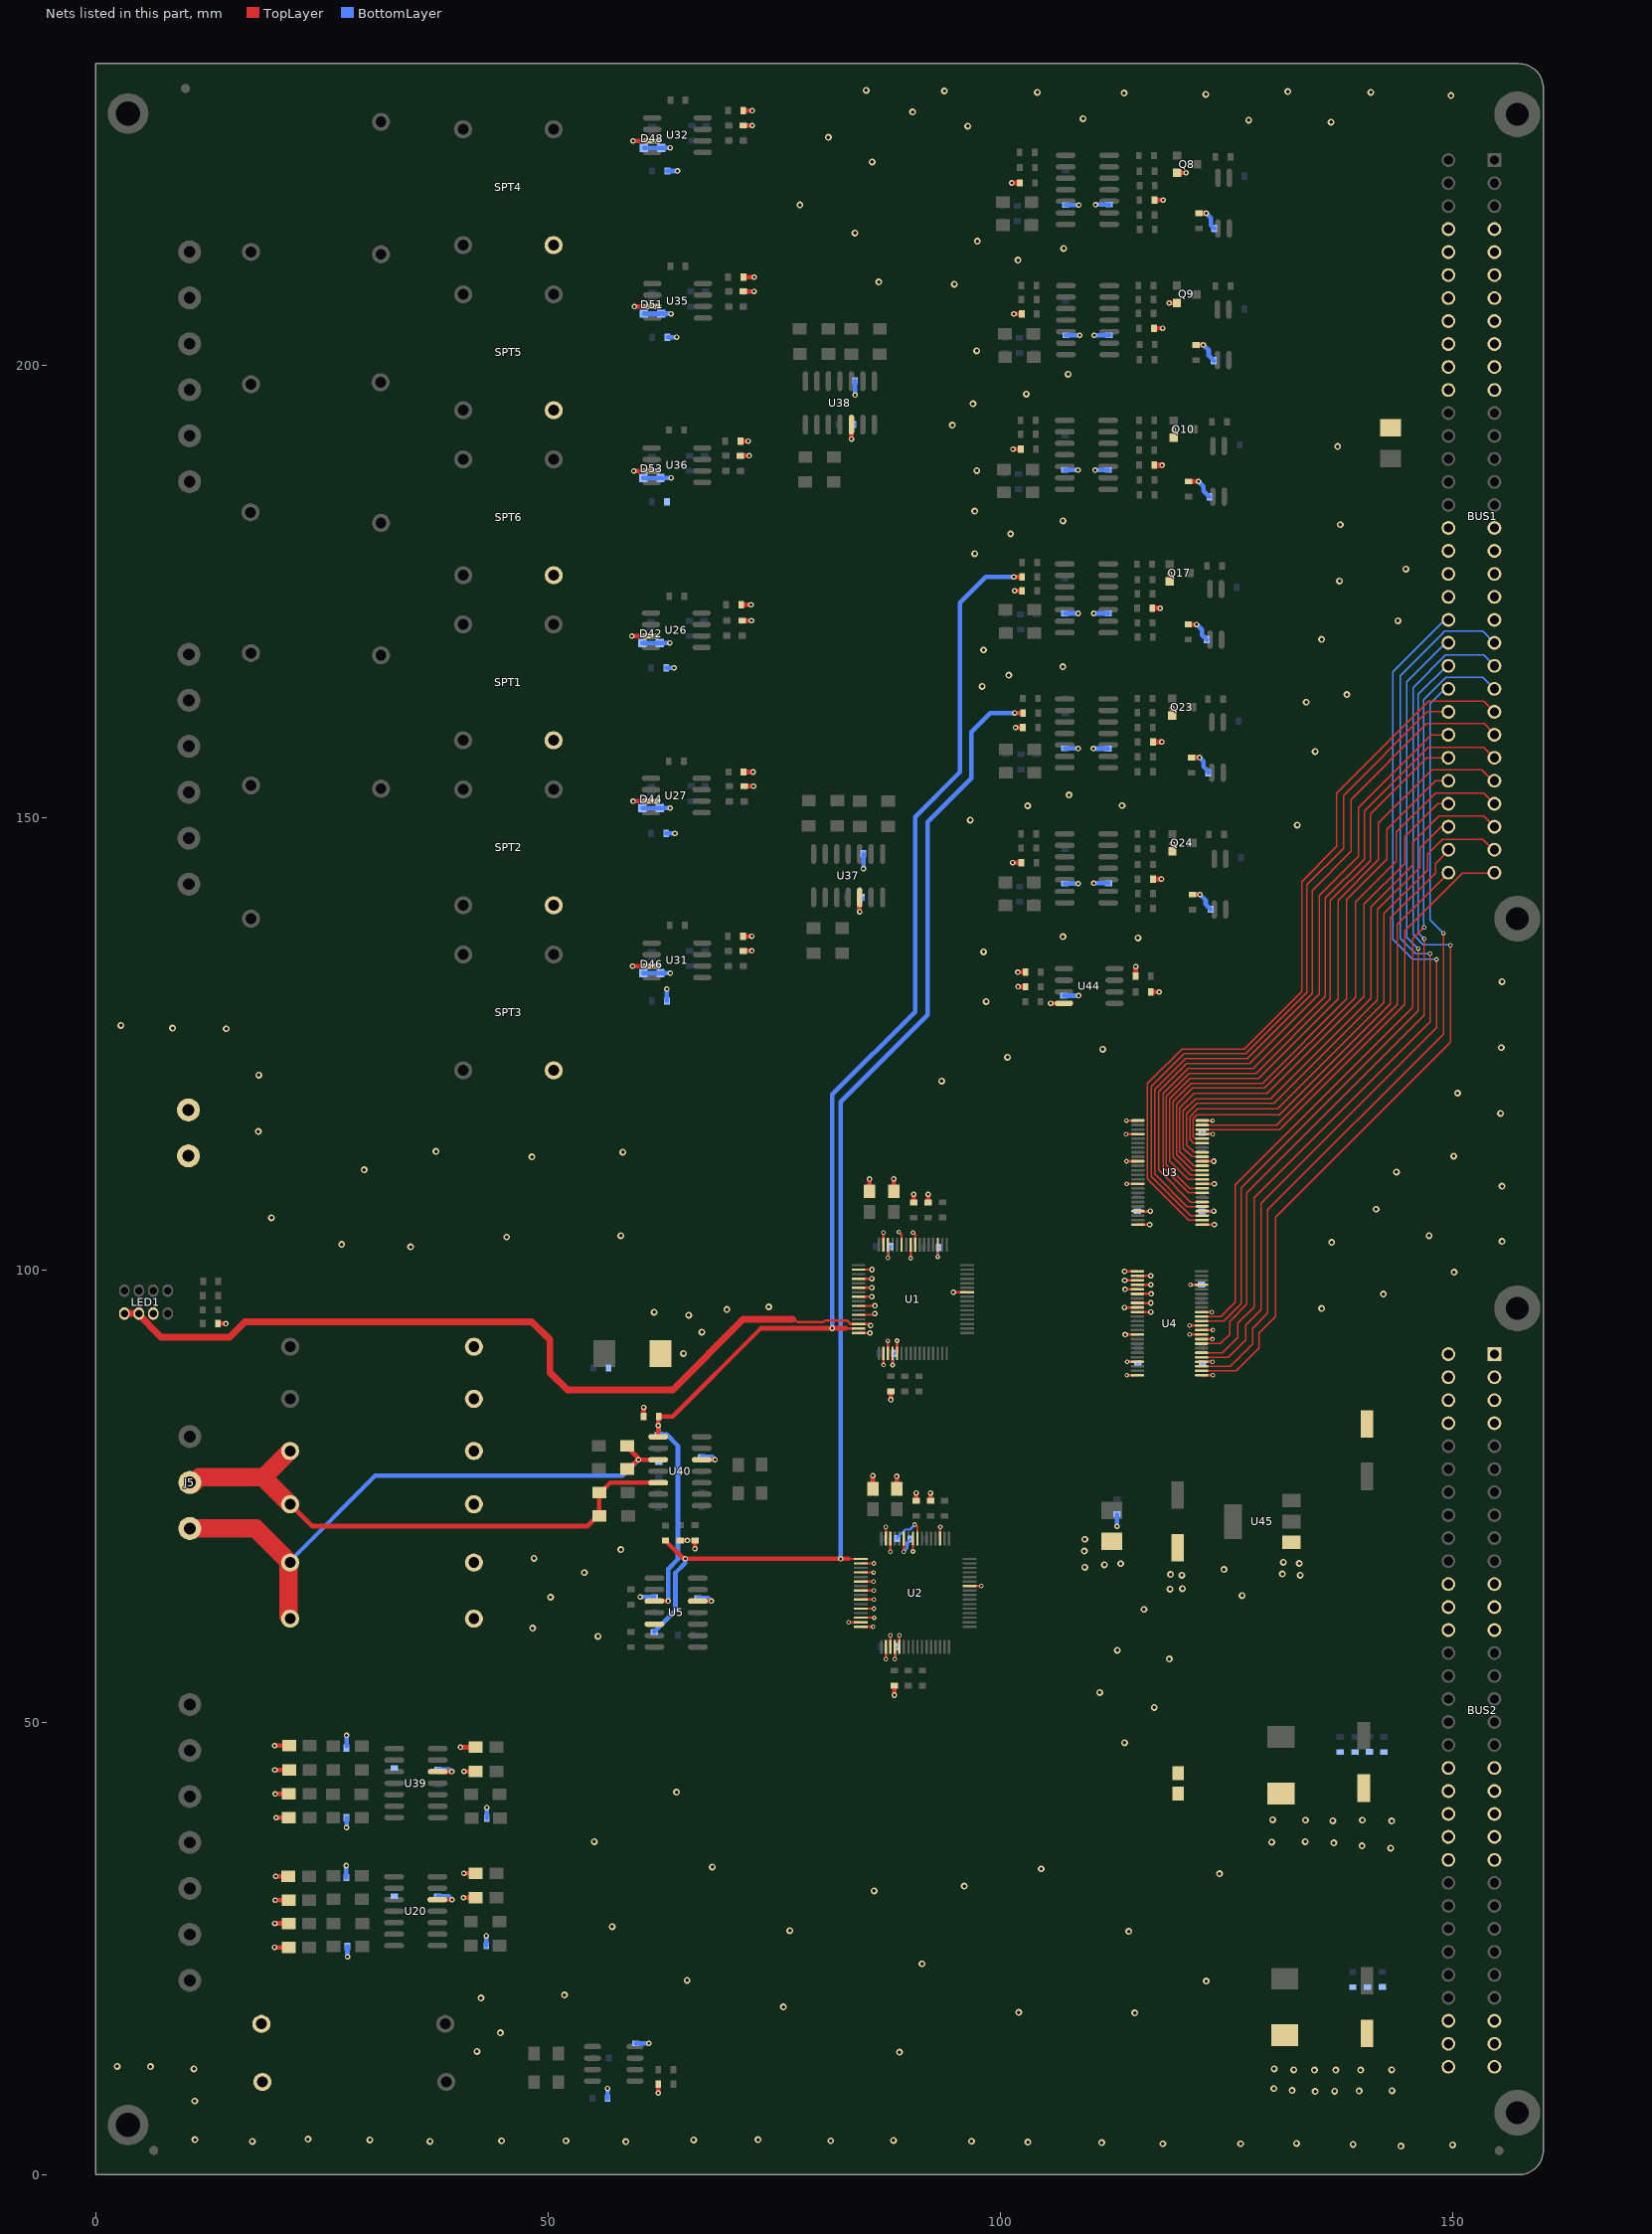
[diagram p0: the nets of this part, all layers, seen from the top]
# Altium PCB MISC80584.PCBDoc (part 4 of 7)
Units mm, origin at the board's own origin, x right, y up, seen from the top; angles counter-clockwise.
Board outline 160.02 x 233.3 mm, 4 copper layers (TopLayer, GND, POWER, BottomLayer); 386 components, 266 nets, 1374 pads, 640 vias.

## Via types
v1: diameter 0.61, hole 0.305, TopLayer to BottomLayer, 342 vias
v2: diameter 0.762, hole 0.381, TopLayer to BottomLayer, 197 vias
v3: diameter 0.508, hole 0.254, TopLayer to BottomLayer, 101 vias

## Nets (pads, with @x,y where several pads share a name; then routed paths per layer and width w, separated by ;. In a path a pad name is that pad's centre, name@x,y a point inside that pad or via, vN(x,y) a via of type N, cw(c..) or ccw(c..) an arc to the next point about the centre after c; other vN are vias at no path point) (continued)
AGND: BUS2.A11 BUS2.A12 BUS2.A13 BUS2.A19 BUS2.A20 BUS2.A21 BUS2.A22 BUS2.A23 BUS2.A30 BUS2.A31 BUS2.A32 BUS2.C11 BUS2.C12 BUS2.C13 BUS2.C19 BUS2.C20 BUS2.C21 BUS2.C22 BUS2.C23 BUS2.C30 BUS2.C31 BUS2.C32 C9.1 C10.1 C11.1 C12.1 C13.1 C14.1 C20.1 C21.1 C23.1 C27.1 C85.1 C93.1 C101.1 C119.2 C120.2 C121.1 C122.1 C123.1 C124.1 C126.1 C136.1 C139.1 C146.2 C147.2 C148.2 C149.1 C173.1 C174.2 C175.2 C176.1 C177.2 C178.1 C179.1 C180.2 C181.2 C182.1 C183.1 C184.2 C192.1 C193.2 C194.1 C195.2 C196.2 C197.1 C204.1 C205.1 C206.2 C215.2 C216.1 C217.1 C218.2 C219.1 C220.1 C224.2 C230.1 C231.2 C232.2 C233.1 C234.2 C235.1 C238.1 C239.2 C240.2 C249.2 C251.1 C252.2 C253.1 C254.2 C255.2 C256.1 C257.1 C261.1 C262.2 CT2.2 CT3.1 CT4.2 CT7.2 CT13.1 D42.1 D42.2 D44.1 D44.2 D46.1 D46.2 D48.1 D48.2 D51.1 D51.2 D53.1 D53.2 J4.1 J4.2 L1.2 LED1.6 Q8.E Q9.E Q10.E Q17.E Q23.E Q24.E R1.1 R2.1 R3.1 R4.1 R6.1 R7.1 R8.1 R9.1 R23.2 R24.2 R25.2 R26.2 R27.2 R29.2 R30.2 R31.2 R32.2 R35.2 R36.2 R38.2 R341.2 R399.2 R400.2 R401.2 R423.2 R430.2 R431.2 R435.2 R437.2 R438.2 R444.2 R445.2 R446.2 SPT1.2 SPT2.2 SPT3.2 SPT4.2 SPT5.2 SPT6.2 U1.43 U1.46 U1.47 U2.43 U2.46 U2.47 U5.5 U5.12 U20.12 U26.3 U27.3 U31.3 U32.3 U35.3 U36.3 U37.12 U38.12 U39.12 U40.12 U44.4 | length 161.6
  TopLayer w0.254: U1.47@87.089,102.805 v3(87.089,104.157) ; U2.47@87.343,70.344 v3(87.343,71.636) ; v3(87.589,101.355) U1.46@87.589,102.805 ; v3(87.843,68.894) U2.46@87.843,70.344 ; v3(88.798,104.191) 89.089,103.901 U1.43@89.089,102.805 ; v3(89.343,68.896) U2.43@89.343,70.344
  TopLayer w0.508: R341.2@13.513,94.082 v1(14.402,94.082) ; v1(19.787,25.171) R30.2@21.336,25.171 ; v1(19.787,47.447) R24.2@21.387,47.447 ; v1(19.812,27.813) R31.2@21.336,27.813 ; v1(19.812,44.755) R23.2@21.387,44.755 ; v1(19.863,30.378) R25.2@21.336,30.378 ; v1(19.863,42.113) R27.2@21.361,42.113 ; v1(19.914,33.02) R26.2@21.311,33.02 ; v1(19.939,39.497) R29.2@21.361,39.497 ; U20.12@37.782,30.429 v1(39.395,30.429) ; U39.12@37.808,44.577 v1(39.37,44.577) ; v1(40.335,47.269) R32.2@42.012,47.269 ; v1(40.665,30.658) R36.2@42.012,30.658 ; v1(40.691,33.35) R38.2@42.012,33.35 ; v1(40.716,44.602) R35.2@42.012,44.602 ; v1(59.258,170.078) U26.3@61.392,170.078 ; v1(59.36,133.604) U31.3@61.468,133.604 ; v1(59.411,151.816) U27.3@61.392,151.816 ; v1(59.411,224.79) U32.3@61.519,224.79 ; v1(59.487,188.316) U36.3@61.468,188.316 ; v1(59.563,206.477) U35.3@61.544,206.477 ; C10.1@60.579,83.82 v1(60.579,84.836) ; v1(62.205,9.068) C9.1@62.205,10.058 ; C11.1@64.618,70.129 v1(65.405,70.129) ; v1(66.243,69.215) C14.1@66.243,70.129 ; U5.12@66.56,63.424 v1(68.047,63.424) ; U40.12@66.992,79.045 v1(68.478,79.045) ; C136.1@71.272,189.992 v1(72.238,189.992) ; C181.2@71.272,191.618 v1(72.136,191.618) ; C180.2@71.374,173.533 v1(72.441,173.533) ; C85.1@71.476,171.78 v1(72.492,171.78) ; C178.1@71.552,136.906 v1(72.542,136.906) ; C101.1@71.577,135.28 v1(72.542,135.28) ; C139.1@71.577,226.492 v1(72.568,226.492) ; C183.1@71.577,228.117 v1(72.568,228.117) ; C126.1@71.603,208.153 v1(72.771,208.153) ; C184.2@71.603,209.728 v1(72.796,209.728) ; C179.1@71.628,155.042 v1(72.669,155.042) ; C93.1@71.679,153.467 v1(72.72,153.467) ; v1(83.541,191.846) U38.12@83.541,193.434 ; v1(84.455,139.598) U37.12@84.455,141.186 ; C121.1@85.547,108.712 v1(85.547,110.058) ; C123.1@85.903,75.844 v1(85.903,77.292) ; C122.1@88.214,108.712 v1(88.214,110.084) ; C124.1@88.544,75.844 v1(88.544,77.216) ; v1(101.27,220.142) R399.2@102.159,220.142 ; v1(101.371,145.034) R431.2@102.311,145.034 ; v1(101.397,190.729) R401.2@102.26,190.729 ; v1(101.498,205.664) R400.2@102.362,205.664 ; v1(101.575,175.057) R423.2@102.413,175.057 ; v1(101.676,159.969) R430.2@102.489,159.969 ; v1(101.93,132.918) C146.2@102.794,132.918 ; v1(101.956,131.318) C147.2@102.794,131.318 ; v1(105.562,129.489) U44.4@107.036,129.489 ; C149.1@114.96,132.486 v1(114.96,133.528) ; C148.2@116.637,130.734 v1(117.577,130.734) ; R438.2@116.992,204.089 v1(117.958,204.089) ; R437.2@117.043,218.237 v1(118.008,218.237) ; v1(118.669,206.883) Q9.E@119.507,206.883 ; Q17.E@118.72,176.098 v1(118.72,176.962) ; Q23.E@118.999,161.265 v1(118.999,162.077) ; Q24.E@119.024,146.279 v1(119.024,147.117) ; Q10.E@119.151,191.973 v1(119.151,192.837) ; Q8.E@119.558,221.259 v1(120.523,221.259)
  TopLayer w0.635: R444.2@116.789,173.152 v1(117.678,173.152) ; R446.2@116.865,143.205 v1(117.805,143.205) ; R445.2@116.865,158.369 v1(117.856,158.369) ; R435.2@117.018,188.951 v1(117.881,188.951)
  BottomLayer w0.305: v3@87.579,101.448 87.579,102.286 C119.2@87.884,102.591 ; v3@89.332,68.91 89.687,69.266 89.687,69.901 C120.2@90.068,70.282
  BottomLayer w0.508: C13.1@27.711,32.868 v1(27.711,34.188) ; v1(27.737,38.405) C20.1@27.737,39.497 ; C12.1@27.737,47.396 v1(27.737,48.59) ; v1(27.838,24.105) C21.1@27.838,25.273 ; C192.1@37.821,30.785 39.04,30.785 v1@39.345,30.48 ; C194.1@37.846,44.806 39.141,44.806 v1@39.319,44.628 ; C27.1@43.18,25.349 v1(43.18,26.441) ; C23.1@43.231,39.446 v1(43.231,40.615) ; C195.2@56.591,8.484 v1(56.591,9.576) ; C220.1@59.741,14.554 v1(61.138,14.554) ; v1(60.198,63.881) C177.2@61.747,63.881 ; D44.2@60.452,151.054 v1(63.5,151.054) ; D42.2@60.452,169.316 v1(63.475,169.316) ; D46.2@60.528,132.817 v1(63.525,132.817) ; D53.2@60.528,187.554 v1(63.627,187.554) ; D51.2@60.604,205.689 D51.1@62.509,205.689 62.662,205.689 v1(63.602,205.689) ; D48.2@60.604,224.028 D48.1@62.509,224.028 62.636,224.028 v1(63.5,224.028) ; C254.2@63.068,148.26 v1(64.033,148.26) ; C252.2@63.068,166.548 v1(63.932,166.548) ; C253.1@63.144,129.743 v1(63.144,131.064) ; C261.1@63.195,221.463 v1(64.313,221.463) ; C251.1@63.221,203.098 v1(64.237,203.098) ; C196.2@66.573,63.754 67.666,63.754 v1@67.97,63.449 ; C197.1@66.98,79.35 68.148,79.35 v1@68.428,79.07 ; v1(83.541,191.846) 83.541,193.116 C240.2@83.845,193.421 ; v1(83.947,196.698) C224.2@83.947,198.272 ; v1(84.455,139.598) 84.455,140.741 C262.2@84.76,141.046 ; v1(84.861,144.348) C233.1@84.861,145.999 ; C216.1@107.036,130.327 v1(108.661,130.327) ; C217.1@107.112,157.658 108.585,157.658 v1(108.61,157.632) ; C232.2@107.112,188.417 v1(108.585,188.417) ; C231.2@107.137,142.723 v1(108.61,142.723) ; C218.2@107.137,172.568 v1(108.61,172.568) ; C215.2@107.213,217.703 v1(108.687,217.703) ; C219.1@107.264,203.302 v1(108.788,203.302) ; v1(110.287,157.632) C238.1@111.912,157.632 ; v1(110.338,142.748) C255.2@111.963,142.748 ; v1(110.338,172.568) C256.1@111.938,172.568 ; v1(110.388,203.302) C193.2@112.039,203.302 ; v1(110.49,188.392) 110.515,188.417 C239.2@111.938,188.417 ; v1(110.515,217.729) 110.541,217.754 C257.1@112.039,217.754
  other v2: 144.272,3.2 149.987,3.327 138.989,3.378 117.958,3.454 126.568,3.454 132.74,3.505 111.201,3.581 103.048,3.632 58.598,3.683 17.323,3.708 36.957,3.708 96.825,3.734 44.882,3.785 51.994,3.785 81.255,3.785 88.189,3.835 30.328,3.886 66.116,3.886 10.973,3.912 73.228,3.912 23.47,3.962 10.947,8.179 134.798,9.246 136.957,9.271 139.675,9.296 143.281,9.322 132.258,9.347 130.251,9.55 134.722,11.608 137.084,11.608 139.827,11.608 132.436,11.633 143.256,11.633 10.871,11.735 130.277,11.735 6.071,11.989 2.388,12.014 88.849,13.589 42.164,13.665 44.729,15.723 114.859,17.907 102.032,17.983 76.022,18.567 42.596,19.558 51.816,19.888 122.758,21.438 65.38,21.514 91.338,23.343 114.198,26.924 76.733,27 57.099,27.457 86.055,31.394 96.012,31.928 124.231,33.299 104.521,33.833 68.174,34.036 143.154,36.119 139.979,36.373 136.855,36.703 129.997,36.779 55.118,36.83 133.706,36.83 143.256,39.116 136.754,39.141 133.731,39.218 140.03,39.218 130.099,39.268 64.211,42.316 55.524,59.538 48.311,60.427 50.292,63.856 54.026,66.573 48.463,68.148 58.064,69.113 64.973,90.78 67.005,93.142 65.557,95.021 61.747,95.352 69.774,95.656 135.509,95.758 74.397,95.936 142.342,97.358 150.165,99.771 34.823,102.565 27.203,102.845 136.627,103.073 155.448,103.175 45.441,103.657 58.064,103.81 147.396,103.81 19.431,105.791 141.529,106.731 155.448,109.271 143.789,110.846 29.693,111.074 48.235,112.522 150.114,112.598 58.268,113.03 37.617,113.106 17.983,115.316 155.296,117.323 150.546,119.558 93.523,120.879 18.034,121.539 100.787,123.52 111.328,124.409 155.372,124.587 14.453,126.67 8.509,126.746 2.794,127.051 98.425,129.667 155.448,131.877 98.146,135.179 115.214,136.703 106.934,136.855 132.817,149.174 96.672,149.733 103.022,151.308 113.462,151.333 107.594,152.502 134.798,157.302 133.807,162.763 138.303,163.601 97.993,164.516 100.94,165.735 106.909,166.675 98.146,168.529 135.509,169.697 143.942,171.755 137.49,176.149 144.831,177.47 97.18,179.172 101.143,181.356 137.566,182.372 106.934,182.804 97.18,183.871 97.409,188.341 137.287,191.008 94.691,193.37 96.977,195.732 102.87,196.799 107.493,199.009 97.384,201.574 94.92,208.94 86.563,209.194 101.956,211.607 107.01,212.903 97.46,213.69 83.922,214.605 77.851,217.703 85.827,222.453 81.001,225.171 96.393,226.416 136.55,226.847 127.457,227.076 109.144,227.228 90.297,227.99 149.809,229.794 122.707,229.921 113.69,230.073 104.089,230.149 140.945,230.149 131.775,230.226 93.828,230.302 85.166,230.378
B_AD_BUSY1: BUS1.A24 U4.14 | length 89
  TopLayer w0.152: U4.14@122.25,94.873 124.362,94.873 125.959,96.469 125.959,109.449 145.567,129.057 145.567,136.601 v3(146.837,137.871)
  BottomLayer w0.152: v3(146.837,137.871) 146.787,137.922 146.787,163.017 149.276,165.506 153.34,165.506 BUS1.A24@154.61,164.236
B_AD_BUSY2: BUS1.C24 U4.3 | length 89.4
  TopLayer w0.152: U4.3@122.25,89.373 125.415,89.373 127.889,91.846 127.889,93.548 129.565,95.225 129.565,106.655 148.971,126.06 148.971,137.135 v3@148.996,137.16
  BottomLayer w0.152: v3(148.971,137.236) 147.523,138.684 147.523,162.611 149.149,164.236 BUS1.C24@149.53,164.236
B_AD_CON: BUS1.C21 U4.5 | length 100.4
  TopLayer w0.152: U4.5@122.25,90.373 125.222,90.373 127.127,92.278 127.127,93.955 128.829,95.656 128.829,107.391 148.209,126.771 v3@148.209,134.468
  BottomLayer w0.152: v3(148.209,134.341) 145.593,134.341 143.383,136.55 143.383,166.091 149.149,171.856 BUS1.C21@149.53,171.856
B_AD_CS1: BUS1.C22 U4.13 | length 90.5
  TopLayer w0.152: U4.13@122.25,94.373 124.7,94.373 126.644,96.317 126.644,109.118 146.177,128.651 v3@146.177,135.458
  BottomLayer w0.152: 144.907,136.83 144.907,138.481 ; v3(146.177,135.534) 144.907,136.804 144.907,138.481 ; BUS1.C22@149.53,169.316 149.2,169.316 144.907,165.024 144.907,138.481
B_AD_CS2: BUS1.A23 U4.2 | length 103.5
  TopLayer w0.152: U4.2@122.25,88.873 126.084,88.873 128.626,91.415 128.626,93.066 130.429,94.869 130.429,105.867 149.758,125.197 v3(149.758,135.89)
  BottomLayer w0.152: v3@149.758,135.966 146.761,135.966 145.618,137.109 145.618,164.363 149.225,167.97 149.911,167.97 150.622,167.97 153.416,167.97 BUS1.A23@154.61,166.776
B_AD_D0: BUS1.A25 U3.26 | length 85.5
  TopLayer w0.152: 116.802,121.171 116.815,121.183 ; U3.26@122.314,105.529 120.785,105.529 116.256,110.058 116.256,120.625 116.815,121.183 ; BUS1.A25@154.61,161.696 153.416,162.89 147.345,162.89 137.185,152.73 137.185,146.812 133.325,142.951 133.325,130.785 126.975,124.435 120.066,124.435 116.815,121.183
B_AD_D1: BUS1.C25 U3.27 | length 77.7
  TopLayer w0.152: U3.27@122.314,106.029 121.022,106.029 116.688,110.363 116.688,120.32 120.294,123.927 127.127,123.927 133.909,130.708 133.909,142.596 137.922,146.609 137.922,152.425 147.193,161.696 BUS1.C25@149.53,161.696
B_AD_D2: BUS1.A26 U3.29 | length 80.6
  TopLayer w0.152: U3.29@122.264,107.029 120.657,107.029 117.069,110.617 117.069,119.964 120.498,123.393 127.305,123.393 134.468,130.556 134.468,141.961 138.786,146.279 138.786,152.019 147.142,160.376 153.492,160.376 BUS1.A26@154.432,159.436
B_AD_D3: BUS1.C26 U3.30 | length 72.7
  TopLayer w0.152: U3.30@122.174,107.518 121.031,107.518 117.5,111.049 117.5,119.761 120.574,122.834 127.584,122.834 135.255,130.505 135.255,141.402 139.573,145.72 139.573,151.105 147.625,159.156 BUS1.C26@149.53,159.156
B_AD_D4: BUS1.A27 U3.32 | length 76.1
  TopLayer w0.152: U3.32@122.264,108.529 120.808,108.529 117.983,111.354 117.983,119.532 120.726,122.276 127.94,122.276 135.915,130.251 135.915,141.097 140.233,145.415 140.233,150.749 147.269,157.785 153.416,157.785 BUS1.A27@154.635,156.566
B_AD_D5: BUS1.C27 U3.33 | length 68.7
  TopLayer w0.152: U3.33@122.264,109.029 120.943,109.029 118.339,111.633 118.339,119.202 120.879,121.742 128.27,121.742 136.474,129.946 136.474,140.843 140.894,145.263 140.894,150.393 147.117,156.616 BUS1.C27@149.53,156.616
B_AD_D6: BUS1.A28 U3.35 | length 71.4
  TopLayer w0.152: U3.35@122.264,110.029 120.73,110.029 118.72,112.039 118.72,118.923 120.98,121.183 128.549,121.183 137.338,129.972 137.338,140.868 141.808,145.339 141.808,149.403 147.701,155.296 153.238,155.296 BUS1.A28@154.508,154.026
B_AD_D7: BUS1.C28 U3.36 | length 63.5
  TopLayer w0.152: U3.36@122.149,110.541 121.031,110.541 119.101,112.471 119.101,118.669 121.082,120.65 128.981,120.65 138.303,129.972 138.303,140.945 142.748,145.39 142.748,148.717 148.107,154.076 BUS1.C28@149.53,154.076
B_AD_D8: BUS1.A29 U3.37 | length 66.8
  TopLayer w0.152: U3.37@122.264,111.029 121.229,111.029 119.482,112.776 119.482,118.339 121.26,120.117 129.235,120.117 139.268,130.15 139.268,140.665 143.789,145.186 143.789,148.438 148.082,152.73 153.441,152.73 BUS1.A29@154.508,151.663
B_AD_D9: BUS1.C29 U3.38 | length 58.8
  TopLayer w0.152: U3.38@121.844,111.506 121.437,111.506 119.837,113.106 119.837,117.958 121.387,119.507 129.464,119.507 140.208,130.251 140.208,140.437 144.704,144.932 144.704,147.879 148.361,151.536 BUS1.C29@149.53,151.536
B_AD_D10: BUS1.A30 U3.40 | length 62.3
  TopLayer w0.152: U3.40@122.264,112.529 121.176,112.529 120.218,113.487 120.218,117.602 121.564,118.948 129.87,118.948 140.97,130.048 140.97,140.132 145.593,144.755 145.593,147.269 148.488,150.165 153.441,150.165 BUS1.A30@154.635,148.971
B_AD_D11: BUS1.C30 U3.41 | length 54.5
  TopLayer w0.152: U3.41@122.072,113.03 121.387,113.03 120.599,113.817 120.599,117.297 121.717,118.415 130.277,118.415 141.707,129.845 141.707,139.852 146.38,144.526 146.38,146.685 148.692,148.996 BUS1.C30@149.53,148.996
B_AD_D12: BUS1.A31 U3.43 | length 57.1
  TopLayer w0.152: U3.43@122.264,114.029 121.378,114.029 120.955,114.452 120.955,116.967 121.793,117.805 130.632,117.805 142.418,129.591 142.418,139.395 147.218,144.196 147.218,145.974 148.869,147.625 153.34,147.625 BUS1.A31@154.229,146.736
B_AD_D13: BUS1.C31 U3.44 | length 49.7
  TopLayer w0.152: U3.44@122.264,114.529 121.513,114.529 121.31,114.732 121.31,116.713 121.768,117.17 130.861,117.17 143.129,129.438 143.129,138.938 148.082,143.891 148.082,144.932 BUS1.C31@149.504,146.355
B_AD_D14: BUS1.A32 U3.46 | length 48.8
  TopLayer w0.152: U3.46@122.264,115.529 130.871,115.529 144.729,129.388 144.729,137.516 151.054,143.84 BUS1.A32@154.559,143.84
B_AD_D15: BUS1.C32 U3.47 | length 44
  TopLayer w0.152: U3.47@122.264,116.029 130.558,116.029 143.891,129.362 143.891,138.201 149.53,143.84 BUS1.C32@149.53,143.916
B_AD_RD: BUS1.C23 U4.8 | length 88
  TopLayer w0.152: U4.8@122.25,91.873 124.334,91.873 125.374,92.913 125.374,94.336 127.254,96.215 127.254,108.56 146.863,128.168 v3@146.863,136.601
  BottomLayer w0.152: v3(146.863,136.627) 146.202,137.287 146.202,163.627 149.352,166.776 BUS1.C23@149.53,166.776
B_AD_RST: BUS1.A22 U4.6 | length 101.9
  TopLayer w0.152: U4.6@122.25,90.873 124.553,90.873 126.263,92.583 126.263,94.158 128.041,95.936 128.041,108.001 147.498,127.457 v3(147.498,134.95)
  BottomLayer w0.152: v3(147.498,134.95) 145.898,134.95 144.196,136.652 144.196,165.684 148.692,170.18 149.123,170.612 153.314,170.612 BUS1.A22@154.61,169.316
GND: BUS1.A4 BUS1.A5 BUS1.A6 BUS1.A7 BUS1.A8 BUS1.A9 BUS1.A10 BUS1.A11 BUS1.A17 BUS1.A18 BUS1.A19 BUS1.A20 BUS1.A21 BUS1.C4 BUS1.C5 BUS1.C6 BUS1.C7 BUS1.C8 BUS1.C9 BUS1.C10 BUS1.C11 BUS1.C17 BUS1.C18 BUS1.C19 BUS1.C20 BUS2.A1 BUS2.A2 BUS2.A3 BUS2.A4 BUS2.C1 BUS2.C2 BUS2.C3 BUS2.C4 C1.1 C2.2 C3.2 C7.1 C8.2 C18.2 C19.1 C22.1 C24.2 C25.1 C26.1 C128.2 C129.2 C156.1 C157.2 C158.2 C159.1 C163.2 C164.2 C165.1 C171.2 CT1.2 CT8.2 CT16.2 CT17.2 L1.1 LED1.2 LED1.4 R591.1 R592.1 R593.1 R600.1 R601.1 R602.1 R608.2 R612.2 U1.2 U1.3 U1.4 U1.5 U1.26 U1.35 U1.40 U1.41 U1.50 U1.52 U1.54 U1.56 U1.58 U1.60 U1.62 U1.64 U2.2 U2.3 U2.4 U2.5 U2.26 U2.35 U2.40 U2.41 U2.50 U2.52 U2.54 U2.56 U2.58 U2.60 U2.62 U2.63 U2.64 U3.1 U3.4 U3.10 U3.15 U3.21 U3.24 U3.25 U3.28 U3.34 U3.39 U3.45 U3.48 U4.1 U4.4 U4.9 U4.10 U4.11 U4.12 U4.15 U4.21 U4.25 U4.26 U4.27 U4.28 U4.29 U4.30 U4.32 U4.33 U4.34 U4.39 U4.45 U4.48 U45.1 | length 219.2
  TopLayer w0.254: 77.064,94.539 77.089,94.539 ; 77.267,94.539 77.546,94.259 80.467,94.259 80.645,94.437 83.033,94.437 83.415,94.055 U1.62@84.339,94.055 85.498,94.055 v1(85.674,93.878) ; v3(83.243,61.094) U2.63@84.593,61.094 ; U1.64@84.339,93.055 v1(85.587,93.055) ; U1.60@84.339,95.055 85.987,95.055 v1(86.131,95.199) ; U1.58@84.339,96.055 v1(86.139,96.055) ; U1.56@84.339,97.055 v1(85.8,97.055) ; U1.54@84.339,98.055 v1(85.79,98.055) ; U1.52@84.339,99.055 v1(85.796,99.055) ; U1.50@84.339,100.055 v1(85.822,100.055) ; U2.64@84.593,60.594 v3(85.943,60.594) ; U2.62@84.593,61.594 v3(86.056,61.594) ; U2.60@84.593,62.594 v3(86.022,62.594) ; U2.58@84.593,63.594 v3(86.022,63.594) ; U2.56@84.593,64.594 v3(86.028,64.594) ; U2.54@84.593,65.594 v3(85.993,65.594) ; U2.52@84.593,66.594 v3(85.999,66.594) ; U2.50@84.593,67.594 v3(86.025,67.594) ; v3(87.343,57.006) U2.2@87.343,58.344 ; U2.3@87.843,58.344 v3(87.843,59.649) ; v3(88.343,56.999) U2.4@88.343,58.344 ; U2.5@88.843,58.344 v3(88.843,59.658) ; v3(90.089,101.326) U1.41@90.089,102.805 ; v3(90.343,68.915) U2.41@90.343,70.344 ; v3(90.348,104.165) 90.589,103.925 U1.40@90.589,102.805 ; v3(90.551,71.882) 90.843,71.59 U2.40@90.843,70.344 ; v3(93.089,101.475) U1.35@93.089,102.805 ; U2.35@93.343,70.344 93.343,71.656 v3(93.37,71.628) ; v1(94.799,97.555) U1.26@96.339,97.555 ; U2.26@96.593,65.094 v3(97.911,65.094) ; v3(113.976,88.373) U4.48@115.15,88.373 ; v3(114.028,89.873) U4.45@115.15,89.873 ; U4.1@122.25,88.373 v3(123.489,88.373) ; U4.4@122.25,89.873 v3(123.452,89.873)
  TopLayer w0.279: v3(87.089,89.518) U1.2@87.089,90.805 ; U1.3@87.589,90.805 v3(87.589,92.193) ; v3(88.089,89.511) U1.4@88.089,90.805 ; U1.5@88.589,90.805 v3(88.589,92.195) ; v1(113.729,95.873) U4.33@115.15,95.873 ; v1(113.741,99.873) U4.25@115.15,99.873 ; v1(113.751,98.873) U4.27@115.15,98.873 ; v1(113.799,97.873) U4.29@115.15,97.873 ; v1(113.802,92.873) U4.39@115.15,92.873 ; v3(113.876,115.029) U3.4@115.214,115.029 ; v3(113.934,112.029) U3.10@115.214,112.029 ; v3(113.938,116.529) U3.1@115.214,116.529 ; v3(113.966,109.529) U3.15@115.214,109.529 ; U4.34@115.15,95.373 v1(116.641,95.373) ; U4.32@115.15,96.373 v1(116.642,96.373) ; U4.30@115.15,97.373 v1(116.673,97.373) ; U4.28@115.15,98.373 v1(116.635,98.373) ; U4.26@115.15,99.373 v1(116.629,99.373) ; U3.24@115.214,105.029 v1(116.51,105.029) ; U3.21@115.214,106.529 v1(116.585,106.529) ; v3(120.91,93.873) U4.12@122.25,93.873 ; v3(120.914,92.873) U4.10@122.25,92.873 ; v3(121.007,98.373) U4.21@122.25,98.373 ; U4.9@122.25,92.373 v3(123.451,92.373) ; U4.11@122.25,93.373 v3(123.518,93.373) ; U4.15@122.25,95.373 v3(123.389,95.373) ; U3.25@122.314,105.029 v1(123.647,105.029) ; U3.28@122.314,106.529 v1(123.595,106.529) ; U3.34@122.314,109.529 v1(123.643,109.529) ; U3.39@122.314,112.029 v1(123.586,112.029) ; U3.45@122.314,115.029 v3(123.487,115.029) ; U3.48@122.314,116.529 v3(123.463,116.529)
  TopLayer w0.508: v1(87.909,85.674) R608.2@87.909,86.589 ; v1(88.29,53.035) R612.2@88.29,54.077 ; C19.1@90.424,107.467 v1(90.424,108.382) ; C25.1@90.703,74.524 v1(90.703,75.387) ; C22.1@92.024,107.467 v1(92.024,108.382) ; C26.1@92.278,74.524 v1(92.278,75.387) ; R600.1@120.777,171.348 v1(121.691,171.348) ; R593.1@120.802,187.147 v1(121.895,187.147) ; R601.1@121.133,156.642 v1(122.022,156.642) ; R602.1@121.26,141.503 v1(122.072,141.503) ; R592.1@121.615,202.235 v1(122.428,202.235) ; R591.1@121.971,216.789 v1(122.758,216.789)
  TopLayer w0.762: LED1.2@3.175,95.199 4.648,95.199 7.239,92.608 14.834,92.608 16.535,94.31 48.209,94.31 50.216,92.304 50.216,88.697 52.146,86.766 63.805,86.766 71.577,94.539 77.064,94.539
  BottomLayer w0.254: v1(86.139,96.055) v1@86.157,96.037 ; v3(87.343,57.006) v3@87.351,56.998 ; v3@88.367,57.023 88.367,58.217 C129.2@88.519,58.369 ; C24.2@88.595,70.333 88.595,70.434 89.484,71.323 90.018,71.323 v3@90.5,71.806 ; v3(93.089,101.475) 93.089,102.436 C18.2@93.116,102.464 ; v3@114.148,89.891 115.062,89.891 C1.1@115.189,89.764 ; C2.2@122.326,89.764 122.428,89.865 v3@123.469,89.865
  BottomLayer w0.279: v3@88.113,89.637 88.113,90.627 C128.2@88.265,90.78 ; v1@113.716,95.86 v1(113.729,95.873) ; v1@113.741,98.882 v1(113.751,98.873) ; v1@113.767,97.841 v1(113.799,97.873) ; v1@113.792,92.862 v1(113.802,92.873) ; v3@113.944,109.55 v3(113.966,109.529) ; C8.2@115.164,106.502 115.189,106.528 v1@116.586,106.528 ; v1(116.641,95.373) v1@116.662,95.352 ; v1(116.673,97.373) v1@116.688,97.358 ; v3@121.006,98.4 C171.2@122.25,98.4 ; C7.1@122.276,106.477 v1@123.571,106.477 ; C165.1@122.276,115.138 122.377,115.037 v3@123.393,115.037 ; v3(123.389,95.373) v3@123.393,95.377 ; v1(123.586,112.029) v1@123.596,112.039 ; v1(123.595,106.529) v1@123.596,106.528 ; v1(123.643,109.529) v1@123.647,109.525
  BottomLayer w0.508: v1(87.909,85.674) v1@87.935,85.649 ; v1(112.903,71.679) C3.2@112.903,72.974 ; v1@121.742,171.323 122.301,170.764 122.301,170.18 C159.1@122.809,169.672 ; v1@121.92,187.147 122.453,186.614 122.453,186.131 C158.2@123.114,185.471 ; v1@122.022,156.667 122.453,156.235 122.453,155.651 122.987,155.118 C163.2@122.987,154.965 ; v1@122.098,141.478 122.707,140.868 122.707,140.411 C164.2@123.241,139.878 ; v1@122.53,202.159 123.038,201.651 123.038,201.041 C157.2@123.596,200.482 ; v1@122.809,216.764 123.292,216.281 123.292,215.468 C156.1@123.647,215.113
  other v2: 113.741,47.777 117.018,51.664 110.998,53.315 118.669,57.023 112.928,57.988 115.875,62.509 126.721,64.033 118.77,64.745 120.142,64.795 120.066,66.294 133.147,66.294 118.821,66.37 131.166,66.421 124.714,66.929 109.347,67.158 111.506,67.437 113.309,67.564 133.045,67.589 131.293,67.716 109.296,68.961 109.347,70.256
ICA: C10.2 R97.1 R349.2 U1.63 U5.3 U40.1 | length 144.7
  TopLayer w0.254: 82.956,93.548 U1.63@83.82,93.548
  TopLayer w0.508: U5.3@61.76,63.424 v1(63.297,63.424) ; U40.1@62.192,81.585 62.192,83.655 62.192,83.706 62.306,83.82 63.779,83.82 73.533,93.574 v1(81.432,93.574) 82.956,93.574 ; v1(101.498,176.606) R349.2@102.413,176.606
  BottomLayer w0.508: v1@62.205,82.753 R97.1@62.205,81.839 63.124,81.839 64.364,80.599 64.364,78.664 64.364,77.622 64.364,68.047 ; v1(63.297,63.424) 63.297,63.576 63.297,66.98 64.364,68.047 ; 64.389,68.072 64.364,68.047 ; v1(81.432,93.574) 81.432,119.405 90.576,128.549 90.576,150.089 95.529,155.042 95.529,173.736 98.4,176.606 v1(101.498,176.606)
  other v1: 62.205,82.829
ICAIN: D60.K D61.A J5.3 R1.2 R2.2 U40.3 | length 67.7
  TopLayer w0.508: D61.A@58.166,78.029 D61.A@58.776,78.029 ; D60.K@58.776,80.594 58.776,80.416 v1@60.096,79.096 ; D61.A@59.182,78.308 59.919,79.045 v1(60.02,79.045) U40.3@62.192,79.045
  TopLayer w2.032: J5.3@10.414,71.45 17.704,71.45 21.311,67.843 R1.2@21.311,61.773
  BottomLayer w0.508: R2.2@21.514,67.869 30.912,77.267 58.242,77.267 v1(60.02,79.045) ; v1@59.944,78.969 v1(60.02,79.045) ; v1@60.046,79.019 v1(60.02,79.045)
ICB: R5.1 R28.1 R350.2 U2.49 | length 135.9
  TopLayer w0.254: 83.236,68.094 U2.49@84.593,68.094
  TopLayer w0.508: R5.1@62.992,70.104 64.999,68.097 v1(82.347,68.097) 83.236,68.097 ; v1(101.6,161.569) R350.2@102.514,161.569
  BottomLayer w0.508: R28.1@61.747,60.02 63.665,61.938 ; 63.652,61.951 64.084,62.382 64.084,66.548 65.176,67.64 v1(65.176,68.123) ; v1(82.347,68.097) 82.347,118.593 91.948,128.194 91.948,149.504 96.799,154.356 96.799,159.461 98.908,161.569 v1(101.6,161.569)
ICBIN: D94.K D96.A J5.2 R3.2 R4.2 U40.5 | length 61.4
  TopLayer w0.508: R3.2@21.438,74.219 23.952,71.704 54.356,71.704 55.677,73.025 55.677,75.311 D96.A@56.096,75.73 ; D96.A@56.109,75.717 56.896,76.505 59.258,76.505 U40.5@62.192,76.505
  TopLayer w2.032: J5.2@10.414,76.53 J5.2@10.897,76.53 ; J5.2@10.744,76.378 J5.2@10.897,76.53 ; 18.741,76.886 R3.2@21.497,74.129 ; R4.2@21.234,79.781 18.593,77.14 11.506,77.14 J5.2@10.897,76.53